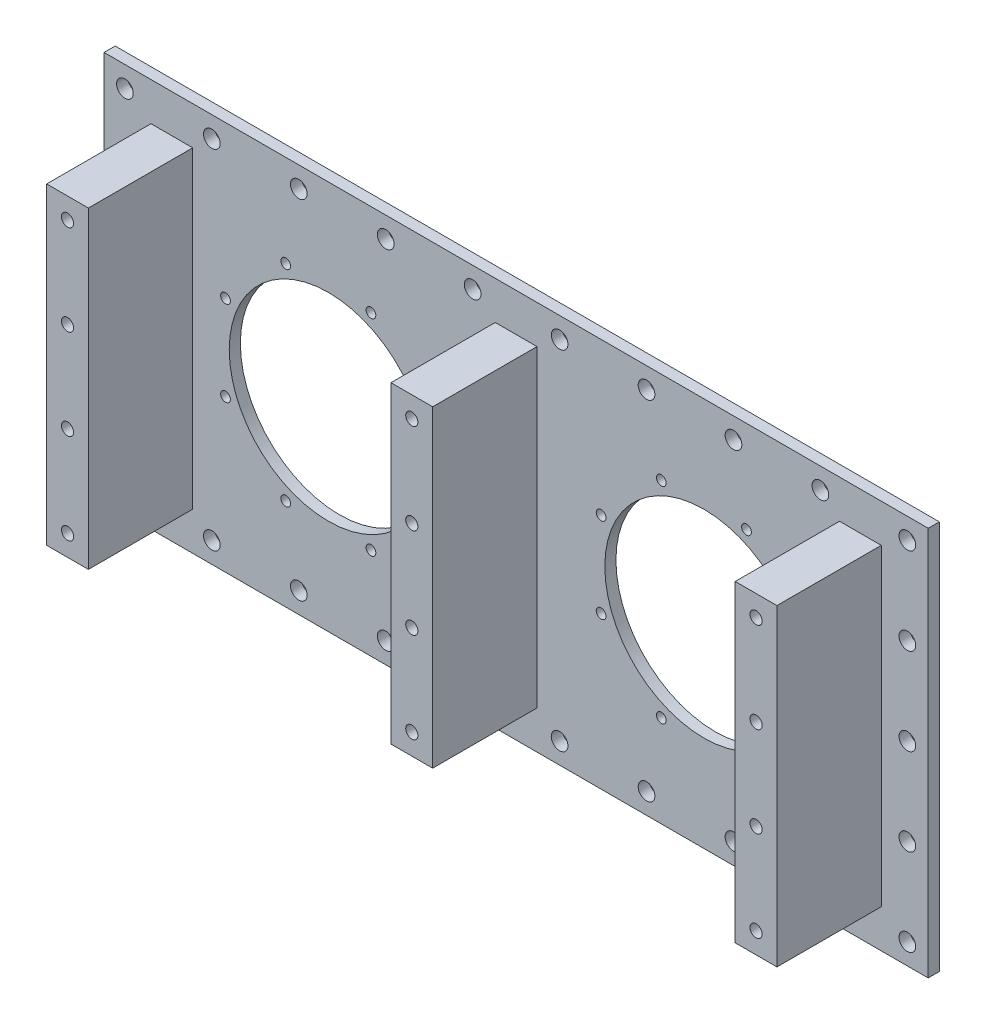
from build123d import *

# Parameters (mm, degrees)
SKETCH1_W           = 1185
SKETCH1_H           = 560
BOSS_EXTRUDE1_DEPTH = 16
SKETCH2_R           = 12
CUT_EXTRUDE1_DEPTH  = 32
SKETCH3_R           = 142.5
CUT_EXTRUDE2_DEPTH  = 32
SKETCH4_W           = 60
SKETCH4_H           = 450
BOSS_EXTRUDE2_DEPTH = 150
LPATTERN1_COUNT     = 4
LPATTERN1_PITCH     = 130
LPATTERN2_COUNT     = 3
LPATTERN2_PITCH     = 495
CIRPATTERN1_COUNT   = 8


with BuildPart() as part:
    # Sketch1 → Boss-Extrude1 (new body)
    with BuildSketch(Plane.XY):
        with Locations((160.973053892, -8.233532934)):
            Rectangle(SKETCH1_W, SKETCH1_H)
    extrude(amount=BOSS_EXTRUDE1_DEPTH)

    # Sketch2 → Cut-Extrude1 (cut)
    with BuildSketch(Plane.XY.offset(16)):
        with Locations((-401.526946108, 241.766467066)):
            Circle(SKETCH2_R)
        with Locations((-276.526946108, 241.766467066)):
            Circle(SKETCH2_R)
        with Locations((-151.526946108, 241.766467066)):
            Circle(SKETCH2_R)
        with Locations((-26.526946108, 241.766467066)):
            Circle(SKETCH2_R)
        with Locations((98.473053892, 241.766467066)):
            Circle(SKETCH2_R)
        with Locations((223.473053892, 241.766467066)):
            Circle(SKETCH2_R)
        with Locations((348.473053892, 241.766467066)):
            Circle(SKETCH2_R)
        with Locations((473.473053892, 241.766467066)):
            Circle(SKETCH2_R)
        with Locations((598.473053892, 241.766467066)):
            Circle(SKETCH2_R)
        with Locations((723.473053892, 241.766467066)):
            Circle(SKETCH2_R)
        with Locations((723.473053892, -258.233532934)):
            Circle(SKETCH2_R)
        with Locations((598.473053892, -258.233532934)):
            Circle(SKETCH2_R)
        with Locations((473.473053892, -258.233532934)):
            Circle(SKETCH2_R)
        with Locations((348.473053892, -258.233532934)):
            Circle(SKETCH2_R)
        with Locations((223.473053892, -258.233532934)):
            Circle(SKETCH2_R)
        with Locations((98.473053892, -258.233532934)):
            Circle(SKETCH2_R)
        with Locations((-26.526946108, -258.233532934)):
            Circle(SKETCH2_R)
        with Locations((-151.526946108, -258.233532934)):
            Circle(SKETCH2_R)
        with Locations((-276.526946108, -258.233532934)):
            Circle(SKETCH2_R)
        with Locations((-401.526946108, -258.233532934)):
            Circle(SKETCH2_R)
        with Locations((-401.526946108, 116.766467066)):
            Circle(SKETCH2_R)
        with Locations((-401.526946108, -8.233532934)):
            Circle(SKETCH2_R)
        with Locations((-401.526946108, -133.233532934)):
            Circle(SKETCH2_R)
        with Locations((723.473053892, -133.233532934)):
            Circle(SKETCH2_R)
        with Locations((723.473053892, -8.233532934)):
            Circle(SKETCH2_R)
        with Locations((723.473053892, 116.766467066)):
            Circle(SKETCH2_R)
    extrude(amount=-CUT_EXTRUDE1_DEPTH, mode=Mode.SUBTRACT)

    # Sketch3 → Cut-Extrude2 (cut)
    with BuildSketch(Plane.XY.offset(16)):
        with Locations((-109.026946108, -8.233532934)):
            Circle(SKETCH3_R)
        with Locations((430.973053892, -8.233532934)):
            Circle(SKETCH3_R)
    extrude(amount=-CUT_EXTRUDE2_DEPTH, mode=Mode.SUBTRACT)

    # Sketch9 → M16 Tapped Hole1 (revolve, cut)
    with BuildSketch(Plane(origin=(-47.797596929, 139.587192268, 16), x_dir=(0, -1, 0), z_dir=(1, 0, 0))):
        Polygon((0, 0), (0, 46.206024333), (7, 42), (7, 0), align=None)
    m16_tapped_hole1 = revolve(axis=Axis((-47.797596929, 139.587192268, 22.35), (0, 0, -1)), mode=Mode.SUBTRACT)

    # CirPattern1: M16 Tapped Hole1 ×8 about axis
    cirpattern1_axis = Axis((-109.026946108, -8.233532934, 0), (0, 0, 1))
    for i in range(1, CIRPATTERN1_COUNT):
        add(m16_tapped_hole1.rotate(cirpattern1_axis, i * 360 / CIRPATTERN1_COUNT), mode=Mode.SUBTRACT)

    # Mirror1: M16 Tapped Hole1 across plane
    add(m16_tapped_hole1.mirror(Plane.ZY.offset(-160.973053892)), mode=Mode.SUBTRACT)

    # Mirror1 copy 1 sketch → Mirror1 copy 1 (revolve, cut)
    with BuildSketch(Plane(origin=(492.202403071, 139.587192268, 16), x_dir=(-0.7071067811865474, -0.7071067811865477, 0), z_dir=(-0.7071067811865477, 0.7071067811865474, 0))):
        Polygon((0, 0), (0, -46.206024333), (7, -42), (7, 0), align=None)
    revolve(axis=Axis((492.202403071, 139.587192268, 22.35), (0, 0, 1)), mode=Mode.SUBTRACT)

    # Mirror1 copy 2 sketch → Mirror1 copy 2 (revolve, cut)
    with BuildSketch(Plane(origin=(578.793779094, 52.995816244, 16), x_dir=(-1, 0, 0), z_dir=(0, 1, 0))):
        Polygon((0, 0), (0, -46.206024333), (7, -42), (7, 0), align=None)
    revolve(axis=Axis((578.793779094, 52.995816244, 22.35), (0, 0, 1)), mode=Mode.SUBTRACT)

    # Mirror1 copy 3 sketch → Mirror1 copy 3 (revolve, cut)
    with BuildSketch(Plane(origin=(578.793779094, -69.462882113, 16), x_dir=(-0.7071067811865477, 0.7071067811865474, 0), z_dir=(0.7071067811865474, 0.7071067811865477, 0))):
        Polygon((0, 0), (0, -46.206024333), (7, -42), (7, 0), align=None)
    revolve(axis=Axis((578.793779094, -69.462882113, 22.35), (0, 0, 1)), mode=Mode.SUBTRACT)

    # Mirror1 copy 4 sketch → Mirror1 copy 4 (revolve, cut)
    with BuildSketch(Plane(origin=(492.202403071, -156.054258136, 16), x_dir=(0, 1, 0), z_dir=(1, 0, 0))):
        Polygon((0, 0), (0, -46.206024333), (7, -42), (7, 0), align=None)
    revolve(axis=Axis((492.202403071, -156.054258136, 22.35), (0, 0, 1)), mode=Mode.SUBTRACT)

    # Mirror1 copy 5 sketch → Mirror1 copy 5 (revolve, cut)
    with BuildSketch(Plane(origin=(369.743704714, -156.054258136, 16), x_dir=(0.7071067811865474, 0.7071067811865478, 0), z_dir=(0.7071067811865478, -0.7071067811865474, 0))):
        Polygon((0, 0), (0, -46.206024333), (7, -42), (7, 0), align=None)
    revolve(axis=Axis((369.743704714, -156.054258136, 22.35), (0, 0, 1)), mode=Mode.SUBTRACT)

    # Mirror1 copy 6 sketch → Mirror1 copy 6 (revolve, cut)
    with BuildSketch(Plane(origin=(283.15232869, -69.462882113, 16), x_dir=(1, 0, 0), z_dir=(0, -1, 0))):
        Polygon((0, 0), (0, -46.206024333), (7, -42), (7, 0), align=None)
    revolve(axis=Axis((283.15232869, -69.462882113, 22.35), (0, 0, 1)), mode=Mode.SUBTRACT)

    # Mirror1 copy 7 sketch → Mirror1 copy 7 (revolve, cut)
    with BuildSketch(Plane(origin=(283.15232869, 52.995816244, 16), x_dir=(0.7071067811865478, -0.7071067811865472, 0), z_dir=(-0.7071067811865472, -0.7071067811865478, 0))):
        Polygon((0, 0), (0, -46.206024333), (7, -42), (7, 0), align=None)
    revolve(axis=Axis((283.15232869, 52.995816244, 22.35), (0, 0, 1)), mode=Mode.SUBTRACT)


with BuildPart() as body_2:
    # Sketch4 → Boss-Extrude2 (new body)
    with BuildSketch(Plane.XY.offset(16)):
        with Locations((-334.026946108, -8.233532934)):
            Rectangle(SKETCH4_W, SKETCH4_H)
    extrude(amount=BOSS_EXTRUDE2_DEPTH)

    # Sketch6 → M20 Tapped Hole1 (revolve, cut)
    with BuildSketch(Plane(origin=(-334.026946108, 186.766467066, 166), x_dir=(0, -1, 0), z_dir=(1, 0, 0))):
        Polygon((0, 0), (0, 55.257530416), (8.75, 50), (8.75, 0), align=None)
    m20_tapped_hole1 = revolve(axis=Axis((-334.026946108, 186.766467066, 172.35), (0, 0, -1)), mode=Mode.SUBTRACT)

    # LPattern1: M20 Tapped Hole1 ×4
    with Locations(*[(0, -i * LPATTERN1_PITCH, 0) for i in range(1, LPATTERN1_COUNT)]):
        add(m20_tapped_hole1, mode=Mode.SUBTRACT)


with BuildPart() as lpattern2_1:
    # LPattern2: pattern copy
    add(body_2.part.moved(Location(Vector(1, 0, 0) * (1 * LPATTERN2_PITCH))))


with BuildPart() as lpattern2_2:
    # LPattern2: pattern copy
    add(body_2.part.moved(Location(Vector(1, 0, 0) * (2 * LPATTERN2_PITCH))))


solid = Compound([part.part, body_2.part, lpattern2_1.part, lpattern2_2.part])
